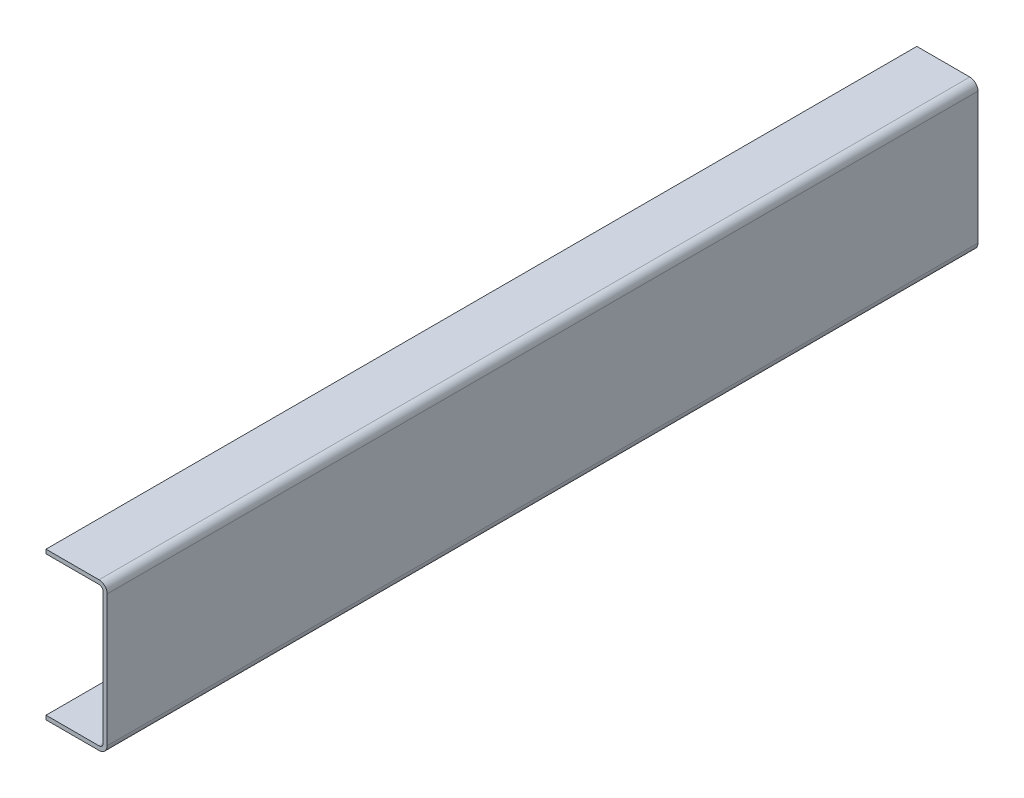
from build123d import *

# Parameters (mm, degrees)
BOSS_EXTRUDE1_DEPTH = 427


with BuildPart() as part:
    # Sketch1 → Boss-Extrude1 (new, symmetric)
    with BuildSketch(Plane.XY):
        with BuildLine():
            Line((-60, -72.5), (-8, -72.5))
            ThreePointArc((-8, -72.5), (-2.343145751, -70.156854249), (0, -64.5))
            Line((0, -64.5), (0, 64.5))
            ThreePointArc((0, 64.5), (-2.343145751, 70.156854249), (-8, 72.5))
            Line((-8, 72.5), (-60, 72.5))
            Line((-60, 72.5), (-60, 68.5))
            Line((-60, 68.5), (-8, 68.5))
            ThreePointArc((-8, 68.5), (-5.171572875, 67.328427125), (-4, 64.5))
            Line((-4, 64.5), (-4, -64.5))
            ThreePointArc((-4, -64.5), (-5.171572875, -67.328427125), (-8, -68.5))
            Line((-8, -68.5), (-60, -68.5))
            Line((-60, -68.5), (-60, -72.5))
        make_face()
    extrude(amount=BOSS_EXTRUDE1_DEPTH, both=True)


solid = part.part
